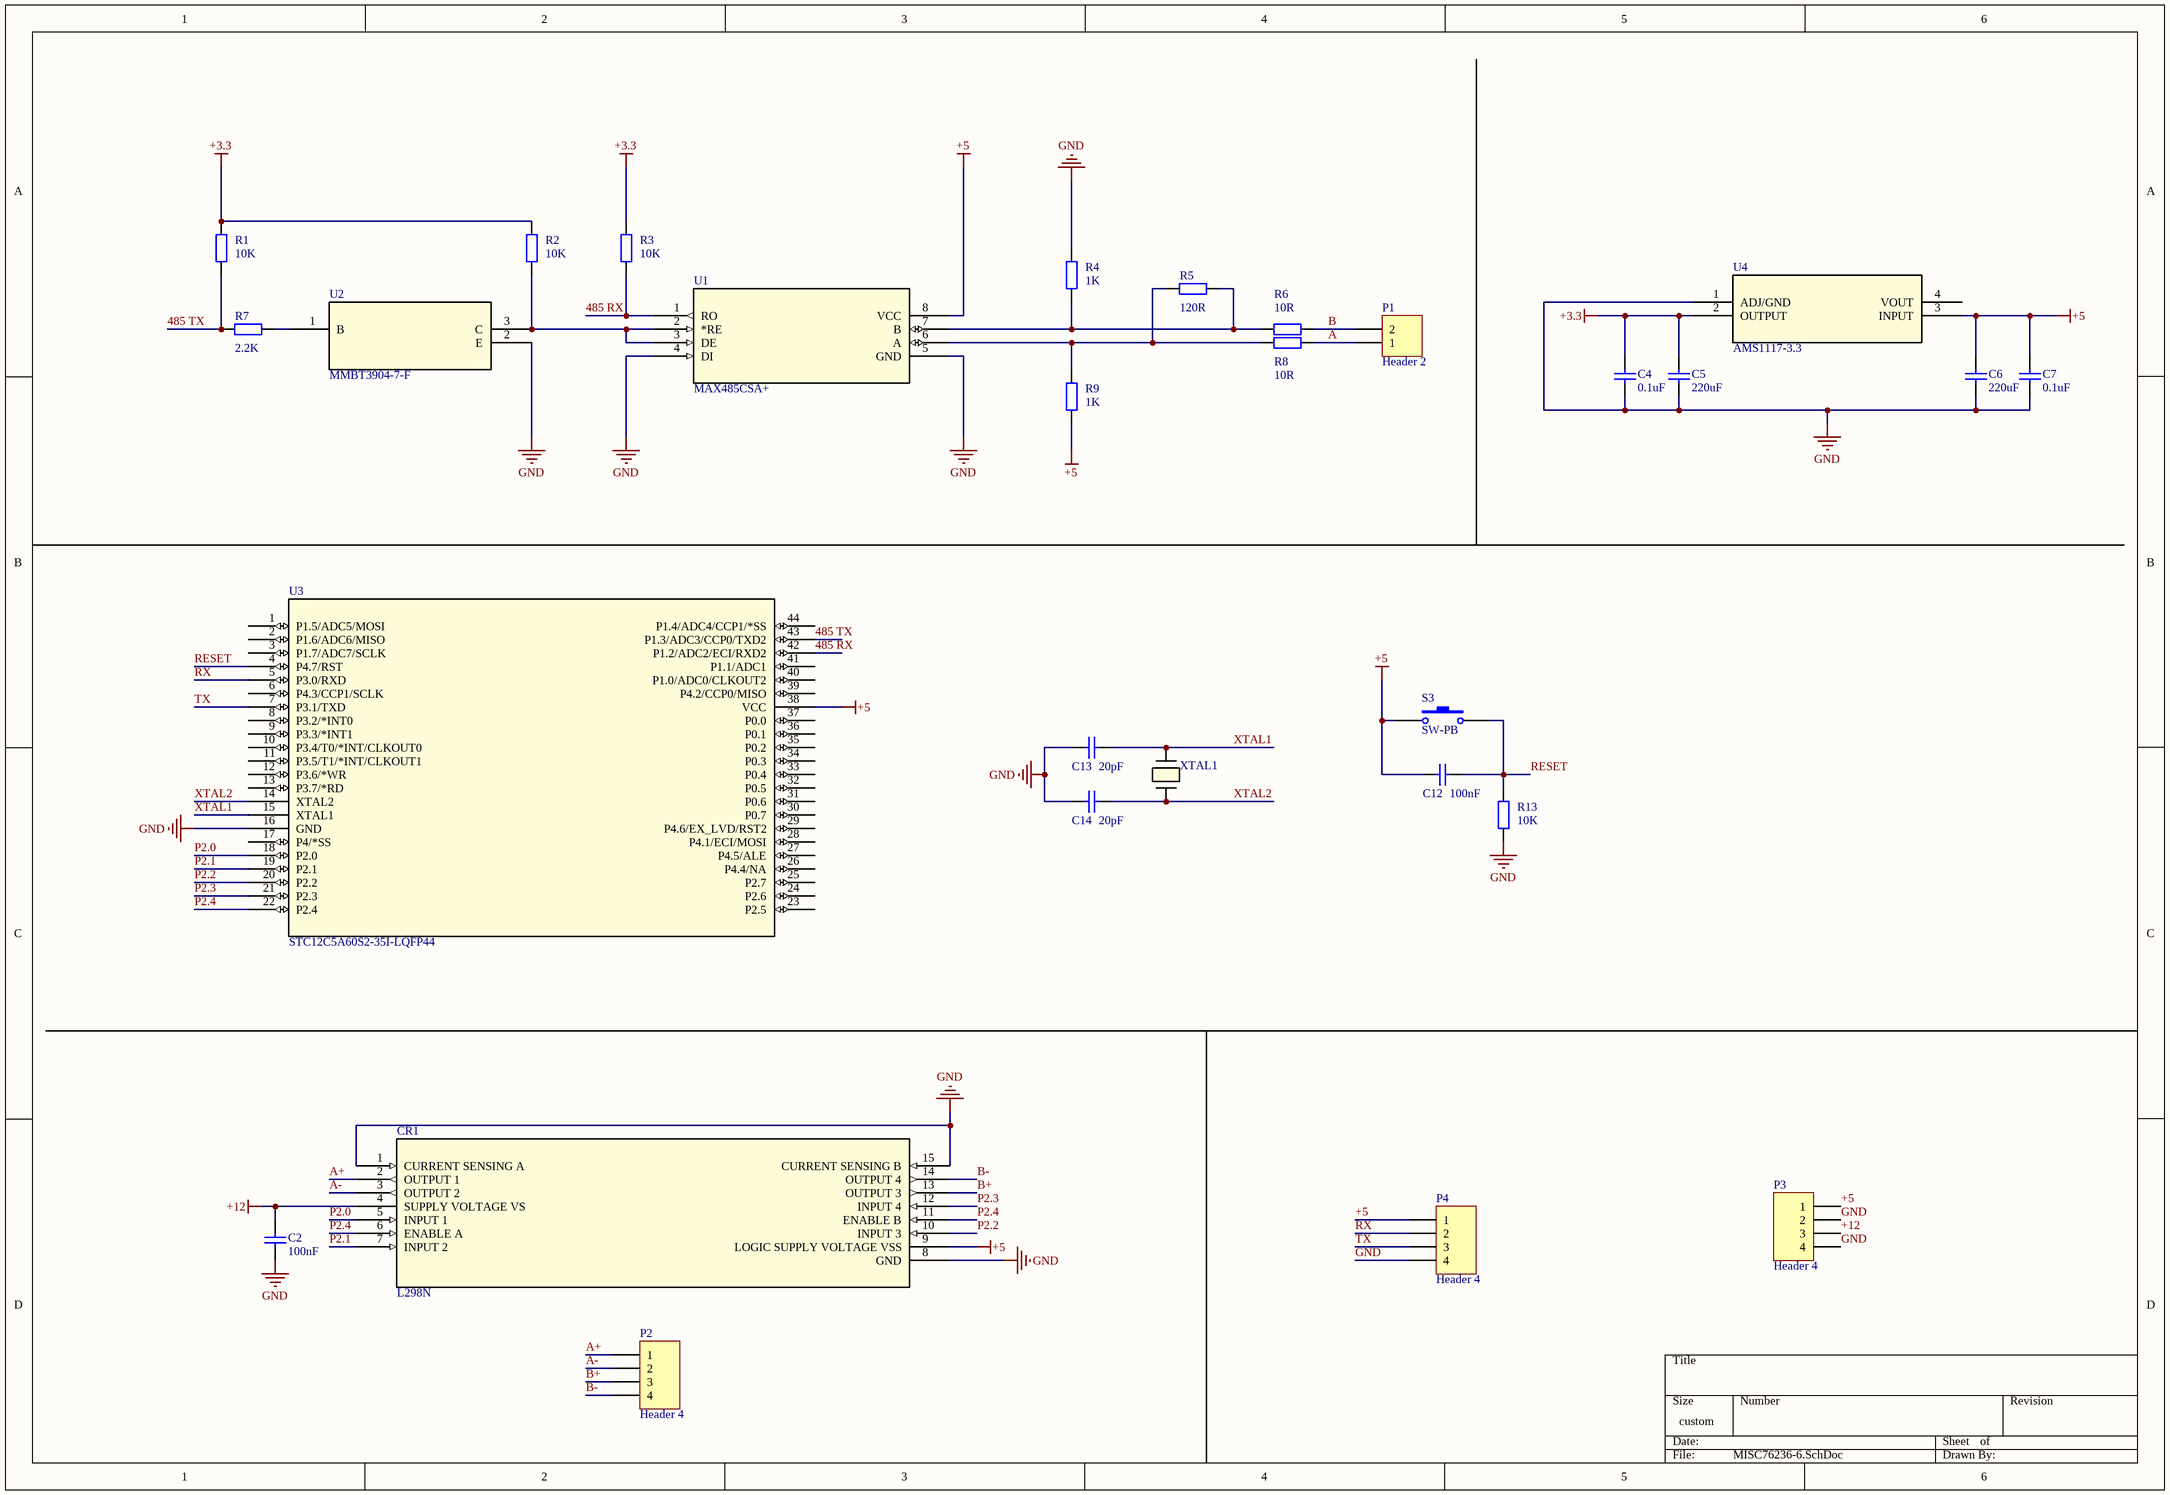
[diagram p0: MISC76236-6.SchDoc]
# Altium project MISC76236-2.PrjPcb
1 sheet, 29 parts. Net scope: global (net labels, ports and power ports of the same name join across sheets).
Board file: MISC76236.PcbDoc

## Sheet MISC76236-6.SchDoc
size 406 x 279 mm

### Parts
C2  value 100nF  [RAD-0.3]  (hidden comment: Cap)
C4  value 0.1uF  [RAD-0.3]  (hidden comment: Cap)
C5  value 220uF  [RAD-0.3]  (hidden comment: Cap)
C6  value 220uF  [RAD-0.3]  (hidden comment: Cap)
C7  value 0.1uF  [RAD-0.3]  (hidden comment: Cap)
C12  value 100nF  [RAD-0.3]  (hidden comment: Cap)
C13  value 20pF  [RAD-0.3]  (hidden comment: Cap)
C14  value 20pF  [RAD-0.3]  (hidden comment: Cap)
CR1  L298N  [Multiwatt15_V_STM]
P1  Header 2  [HDR1X2]
P2  Header 4  [HDR1X4]
P3  Header 4  [HDR1X4]
P4  Header 4  [HDR1X4]
R1  value 10K  [AXIAL-0.4]  (hidden comment: Res2)
R2  value 10K  [AXIAL-0.4]  (hidden comment: Res2)
R3  value 10K  [AXIAL-0.4]  (hidden comment: Res2)
R4  value 1K  [AXIAL-0.4]  (hidden comment: Res2)
R5  value 120R  [AXIAL-0.4]  (hidden comment: Res2)
R6  value 10R  [AXIAL-0.4]  (hidden comment: Res2)
R7  value 2.2K  [AXIAL-0.4]  (hidden comment: Res2)
R8  value 10R  [AXIAL-0.4]  (hidden comment: Res2)
R9  value 1K  [AXIAL-0.4]  (hidden comment: Res2)
R13  value 10K  [AXIAL-0.4]  (hidden comment: Res2)
S3  SW-PB  [SPST-2]
U1  MAX485CSA+  [21-0041B_8_MXM]
U2  MMBT3904-7-F  [SOT-23_1_DIO]
U3  STC12C5A60S2-35I-LQFP44  [LQFP44_STC89_STC_SCM]
U4  AMS1117-3.3  [TS3B_TEX]
XTAL1  HC49S-11.0592-30-50-70-30-ATF  [XTAL_HC49S_MTC]  (value not drawn)

### Nets
+3.3: C4.2 C5.2 R1.2 R2.2 R3.2 U4.2(OUTPUT)
+5: C6.2 C7.2 C12.1 CR1.9(LOGIC_SUPPLY_VOLTAGE_VSS) P3.1 P4.1 R9.1 S3.1 U1.8(VCC) U3.38(VCC) U4.3(INPUT)
+12: C2.2 CR1.4(SUPPLY_VOLTAGE_VS) P3.3
GND: C2.1 C4.1 C5.1 C6.1 C7.1 C13.1 C14.1 CR1.1(CURRENT_SENSING_A) CR1.8(GND) CR1.15(CURRENT_SENSING_B) P3.2 P3.4 P4.4 R4.2 R13.1 U1.4(DI) U1.5(GND) U2.2(E) U3.16(GND) U4.1(ADJ/GND)
485 RX: R3.1 U1.1(RO) U3.42(P1.2/ADC2/ECI/RXD2)
485 TX: R1.1 R7.1 U3.43(P1.3/ADC3/CCP0/TXD2)
A: P1.1 R8.2
A+: CR1.2(OUTPUT_1) P2.1
A-: CR1.3(OUTPUT_2) P2.2
B: P1.2 R6.2
B+: CR1.13(OUTPUT_3) P2.3
B-: CR1.14(OUTPUT_4) P2.4
P2.0: CR1.5(INPUT_1) U3.18(P2.0)
P2.1: CR1.7(INPUT_2) U3.19(P2.1)
P2.2: CR1.10(INPUT_3) U3.20(P2.2)
P2.3: CR1.12(INPUT_4) U3.21(P2.3)
P2.4: CR1.6(ENABLE_A) CR1.11(ENABLE_B) U3.22(P2.4)
RESET: C12.2 R13.2 S3.2 U3.4(P4.7/RST)
RX: P4.2 U3.5(P3.0/RXD)
TX: P4.3 U3.7(P3.1/TXD)
XTAL1: C13.2 U3.15(XTAL1) XTAL1.2
XTAL2: C14.2 U3.14(XTAL2) XTAL1.1
NetR2_1: R2.1 U1.2(*RE) U1.3(DE) U2.3(C)
NetR4_1: R4.1 R5.2 R6.1 U1.7(B)
NetR5_1: R5.1 R8.1 R9.2 U1.6(A)
NetR7_2: R7.2 U2.1(B)

Not connected (* = marked no-connect by the designer): U3 1(P1.5/ADC5/MOSI) 2(P1.6/ADC6/MISO) 3(P1.7/ADC7/SCLK) 6(P4.3/CCP1/SCLK) 8(P3.2/*INT0) 9(P3.3/*INT1) 10(P3.4/T0/*INT/CLKOUT0) 11(P3.5/T1/*INT/CLKOUT1) 12(P3.6/*WR) 13(P3.7/*RD) 17(P4/*SS) 23(P2.5) 24(P2.6) 25(P2.7) 26(P4.4/NA) 27(P4.5/ALE) 28(P4.1/ECI/MOSI) 29(P4.6/EX_LVD/RST2) 30(P0.7) 31(P0.6) 32(P0.5) 33(P0.4) 34(P0.3) 35(P0.2) 36(P0.1) 37(P0.0) 39(P4.2/CCP0/MISO) 40(P1.0/ADC0/CLKOUT2) 41(P1.1/ADC1) 44(P1.4/ADC4/CCP1/*SS); U4 4(VOUT)

### Library data of the parts
C2 C4-C7 C12-C14 = Cap: Capacitor; Published: 8-Jun-2000; LatestRevisionDate: 17-Jul-2002; LatestRevisionNote: Re-released for DXP Platform.; PackageReference: RAD-0.3; PackageDescription: Radial Cap, Thru-Hole; 2 Leads; 0.3 in Pin Spacing; Publisher: Altium Limited
CR1 = L298N: No Description Available; Mfr_Name: STMicroelectronics; RefDes: RefDes; Type: Type
P1 = Header 2: Header, 2-Pin; LatestRevisionDate: 17-Jul-2002; LatestRevisionNote: Re-released for DXP Platform.; Publisher: Altium Limited
P2-P4 = Header 4: Header, 4-Pin; LatestRevisionDate: 17-Jul-2002; LatestRevisionNote: Re-released for DXP Platform.; Publisher: Altium Limited
R1-R9 R13 = Res2: Resistor; Published: 8-Jun-2000; LatestRevisionDate: 17-Jul-2002; LatestRevisionNote: Re-released for DXP Platform.; PackageReference: AXIAL-0.4; PackageDescription: Axial Device, Thru-Hole; 2 Leads; 0.4 in Pin Spacing; Publisher: Altium Limited
S3 = SW-PB: Switch; Published: 24-Mar-1999; LatestRevisionDate: 17-Jul-2002; LatestRevisionNote: Re-released for DXP Platform.; PackageReference: SPST-2; PackageDescription: Switch; 2 Leads; Publisher: Altium Limited
U1 = MAX485CSA+: No Description Available; Mfr_Name: Analog Devices Inc; RefDes: RefDes; Type: Type
U2 = MMBT3904-7-F: No Description Available; Mfr_Name: Diodes Inc; RefDes: RefDes; Type: Type
U3 = STC12C5A60S2-35I-LQFP44: No Description Available; Mfr_Name: STC; Type: Embedded; RefDes: RefDes
U4 = AMS1117-3.3: No Description Available; Mfr_Name: ams OSRAM; RefDes: RefDes; Type: Type
XTAL1 = HC49S-11.0592-30-50-70-30-ATF: No Description Available; Mfr_Name: Multicomp